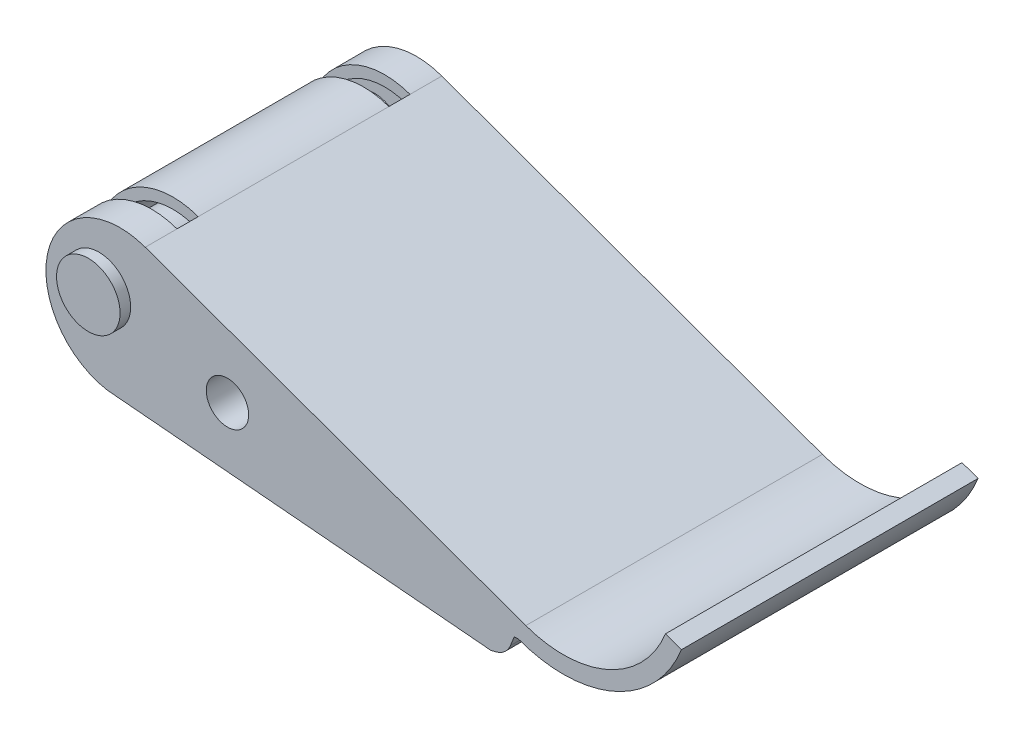
from build123d import *

# Parameters (mm, degrees)
BOSS_EXTRUDE1_DEPTH      = 7
BOSS_EXTRUDE1_DEPTH_BACK = 7
SKETCH1_R                = 1
CUT_EXTRUDE1_DEPTH       = 6
CUT_EXTRUDE1_DEPTH_BACK  = 6
CUT_EXTRUDE2_DEPTH       = 6
CUT_EXTRUDE2_DEPTH_BACK  = 6
SKETCH3_R                = 3
CUT_EXTRUDE3_START       = -1
CUT_EXTRUDE3_DEPTH       = 1
CUT_EXTRUDE4_DEPTH       = 1
BOSS_EXTRUDE2_DEPTH      = 7.5
BOSS_EXTRUDE2_DEPTH_BACK = 7.5
SKETCH6_R                = 1.5
CUT_EXTRUDE5_DEPTH       = 5.5
CUT_EXTRUDE5_DEPTH_BACK  = 5.5


with BuildPart() as part:
    # Sketch1 → Boss-Extrude1 (new, two sides: drawn at the far end of the back side and taken through both)
    with BuildSketch(Plane.XY.offset(-BOSS_EXTRUDE1_DEPTH_BACK)):
        with BuildLine():
            Line((2.892231378, 2.053172864), (21, 0.468948388))
            Line((21, 0.468948388), (21.243569075, 0.530116447))
            ThreePointArc((21.243569075, 0.530116447), (21.657311704, 0.746381181), (21.927791013, 1.126899697))
            Line((21.927791013, 1.126899697), (22.11, 1.58))
            Line((22.11, 1.58), (22.31866709, 1.58))
            ThreePointArc((22.31866709, 1.58), (26.857258232, 1.7173207), (30, 4.994642886))
            Line((30, 4.994642886), (29.24792212, 5.268376848))
            ThreePointArc((29.24792212, 5.268376848), (26.549597889, 2.45607622), (22.654950899, 2.308721878))
            Line((22.654950899, 2.308721878), (4.688013818, 8.792206429))
            ThreePointArc((4.688013818, 8.792206429), (0.118016194, 6.401213367), (2.892231378, 2.053172864))
        make_face()
        with Locations((8.57, 4.38)):
            Circle(SKETCH1_R, mode=Mode.SUBTRACT)
    extrude(amount=BOSS_EXTRUDE1_DEPTH + BOSS_EXTRUDE1_DEPTH_BACK)

    # Sketch2 → Cut-Extrude1 (cut, two sides: drawn at the far end of the back side and taken through both)
    with BuildSketch(Plane.XY.offset(-CUT_EXTRUDE1_DEPTH_BACK)):
        with BuildLine():
            Line((4.63, 0.629363491), (3.5, 5.5))
            Line((3.5, 5.5), (-1.5, 5.5))
            ThreePointArc((-1.5, 5.5), (0.389533797, 1.585284174), (4.63, 0.629363491))
        make_face()
    extrude(amount=CUT_EXTRUDE1_DEPTH + CUT_EXTRUDE1_DEPTH_BACK, mode=Mode.SUBTRACT)

    # Sketch3 → Cut-Extrude2 (cut, two sides: drawn at the far end of the back side and taken through both)
    with BuildSketch(Plane.XY.offset(-CUT_EXTRUDE2_DEPTH_BACK)):
        with Locations((3.5, 5.5)):
            Circle(SKETCH3_R)
    extrude(amount=CUT_EXTRUDE2_DEPTH + CUT_EXTRUDE2_DEPTH_BACK, mode=Mode.SUBTRACT)

    # Sketch4 → Cut-Extrude3 (cut)
    with BuildSketch(Plane.XY.offset(5.5).offset(CUT_EXTRUDE3_START)):
        with BuildLine():
            Line((2.302929498, 2.211075827), (4.697070502, 8.788924173))
            ThreePointArc((4.697070502, 8.788924173), (0.211075827, 6.697070502), (2.302929498, 2.211075827))
        make_face()
    extrude(amount=CUT_EXTRUDE3_DEPTH, mode=Mode.SUBTRACT)

    # Sketch5 → Cut-Extrude4 (cut)
    with BuildSketch(Plane.XY.offset(-5.5)):
        with BuildLine():
            Line((2.302929498, 2.211075827), (4.697070502, 8.788924173))
            ThreePointArc((4.697070502, 8.788924173), (0.211075827, 6.697070502), (2.302929498, 2.211075827))
        make_face()
    extrude(amount=CUT_EXTRUDE4_DEPTH, mode=Mode.SUBTRACT)

    # Sketch6 → Boss-Extrude2 (add, two sides: drawn at the far end of the back side and taken through both)
    with BuildSketch(Plane.XY.offset(-BOSS_EXTRUDE2_DEPTH_BACK)):
        with Locations((2.5, 6)):
            Circle(SKETCH6_R)
    extrude(amount=BOSS_EXTRUDE2_DEPTH + BOSS_EXTRUDE2_DEPTH_BACK)

    # Sketch7 → Cut-Extrude5 (cut, two sides: drawn at the far end of the back side and taken through both)
    with BuildSketch(Plane.XY.offset(-CUT_EXTRUDE5_DEPTH_BACK)):
        Polygon((11.724964743, 1.0104331), (21.686911724, 0.138875672), (21.747920744, 0.836211961), (11.785973763, 1.707769388), align=None)
    extrude(amount=CUT_EXTRUDE5_DEPTH + CUT_EXTRUDE5_DEPTH_BACK, mode=Mode.SUBTRACT)


solid = part.part
